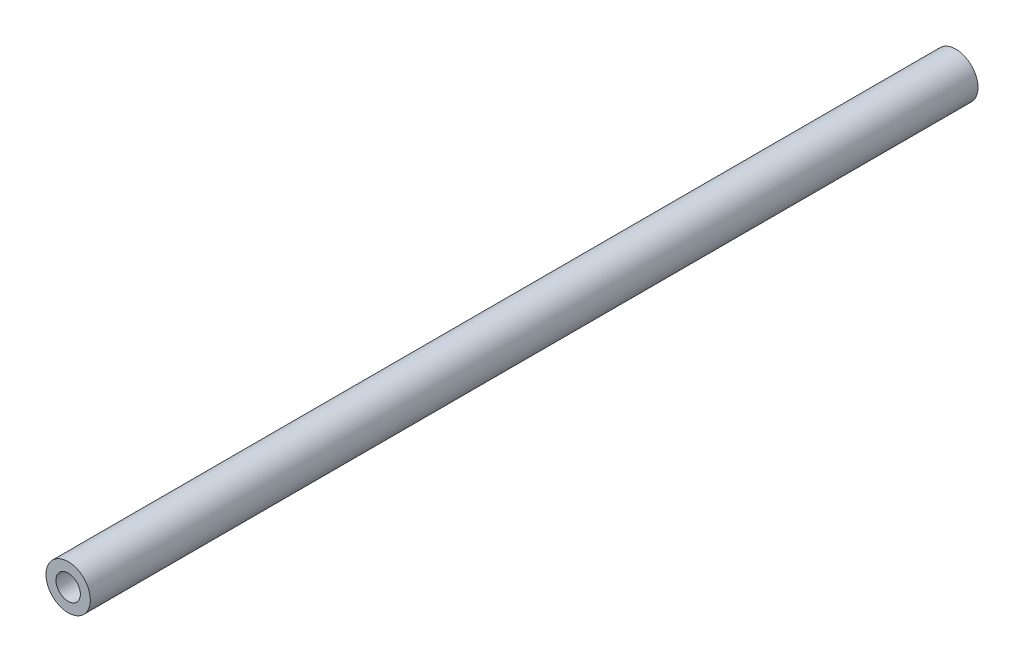
from build123d import *

# Parameters (mm, degrees)
SKETCH1_R             = 3
BOSS_EXTRUDE1_DEPTH   = 60
M4_TAPPED_HOLE1_D     = 3.3
M4_TAPPED_HOLE1_DEPTH = 10.1
M4_TAPPED_HOLE1_TIP   = 0.991420021
M4_TAPPED_HOLE2_D     = 3.3
M4_TAPPED_HOLE2_DEPTH = 10.1
M4_TAPPED_HOLE2_TIP   = 0.991420021


with BuildPart() as part:
    # Sketch1 → Boss-Extrude1 (new, symmetric)
    with BuildSketch(Plane.XY):
        Circle(SKETCH1_R)
    extrude(amount=BOSS_EXTRUDE1_DEPTH, both=True)

    # M4 Tapped Hole1
    with Locations(Plane.XY.offset(60)):
        with Locations((0, 0)):
            Hole(M4_TAPPED_HOLE1_D / 2, depth=M4_TAPPED_HOLE1_DEPTH)
            with Locations((0, 0, -(M4_TAPPED_HOLE1_DEPTH + M4_TAPPED_HOLE1_TIP / 2))):  # 118° drill point
                Cone(0, M4_TAPPED_HOLE1_D / 2, M4_TAPPED_HOLE1_TIP, mode=Mode.SUBTRACT)

    # M4 Tapped Hole2
    with Locations(Plane(origin=(0, 0, -60), x_dir=(-1, 0, 0), z_dir=(0, 0, -1))):
        with Locations((0, 0)):
            Hole(M4_TAPPED_HOLE2_D / 2, depth=M4_TAPPED_HOLE2_DEPTH)
            with Locations((0, 0, -(M4_TAPPED_HOLE2_DEPTH + M4_TAPPED_HOLE2_TIP / 2))):  # 118° drill point
                Cone(0, M4_TAPPED_HOLE2_D / 2, M4_TAPPED_HOLE2_TIP, mode=Mode.SUBTRACT)


solid = part.part
